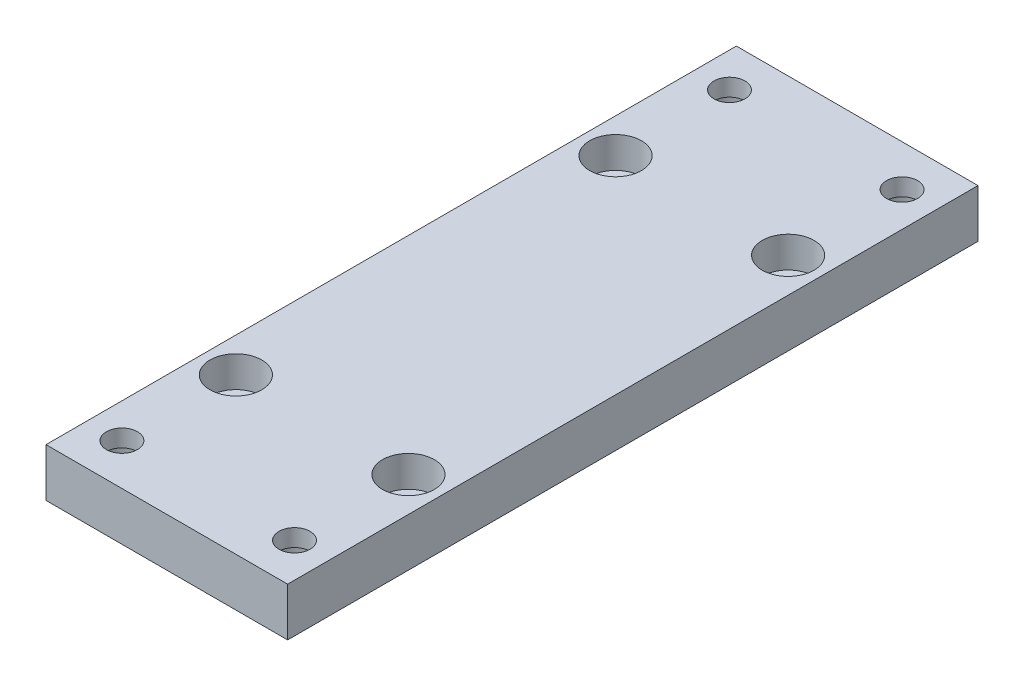
from build123d import *

# Parameters (mm, degrees)
SKETCH1_W                                          = 70
SKETCH1_H                                          = 200
BOSS_EXTRUDE1_DEPTH                                = 14
HOLE_SIZE_BASED_ON_SOCKET_HEAD_CAP_SCR_D           = 9
HOLE_SIZE_BASED_ON_SOCKET_HEAD_CAP_SCR_CBORE_D     = 15
HOLE_SIZE_BASED_ON_SOCKET_HEAD_CAP_SCR_CBORE_DEPTH = 9
HOLE_SIZE_BASED_ON_SOCKET_HEAD_CAP_2_D             = 9
HOLE_SIZE_BASED_ON_SOCKET_HEAD_CAP_2_CBORE_D       = 15
HOLE_SIZE_BASED_ON_SOCKET_HEAD_CAP_2_CBORE_DEPTH   = 9


with BuildPart() as part:
    # Sketch1 → Boss-Extrude1 (new body)
    with BuildSketch(Plane(origin=(0, 0, 0), x_dir=(1, 0, 0), z_dir=(0, 1, 0))):
        with Locations((35, 100)):
            Rectangle(SKETCH1_W, SKETCH1_H)
    extrude(amount=BOSS_EXTRUDE1_DEPTH)

    # Hole size _based on_ socket head cap scr (through all)
    with Locations(Plane(origin=(0, 14, 0), x_dir=(1, 0, 0), z_dir=(0, 1, 0))):
        with Locations((10, 155), (60, 155), (60, 45), (10, 45)):
            CounterBoreHole(HOLE_SIZE_BASED_ON_SOCKET_HEAD_CAP_SCR_D / 2, HOLE_SIZE_BASED_ON_SOCKET_HEAD_CAP_SCR_CBORE_D / 2, HOLE_SIZE_BASED_ON_SOCKET_HEAD_CAP_SCR_CBORE_DEPTH)

    # Hole size _based on_ socket head cap 2 (through all)
    with Locations(Plane(origin=(0, 0, 0), x_dir=(-1, 0, 0), z_dir=(0, -1, 0))):
        with Locations((-60, 188), (-10, 188), (-10, 12), (-60, 12)):
            CounterBoreHole(HOLE_SIZE_BASED_ON_SOCKET_HEAD_CAP_2_D / 2, HOLE_SIZE_BASED_ON_SOCKET_HEAD_CAP_2_CBORE_D / 2, HOLE_SIZE_BASED_ON_SOCKET_HEAD_CAP_2_CBORE_DEPTH)


solid = part.part
